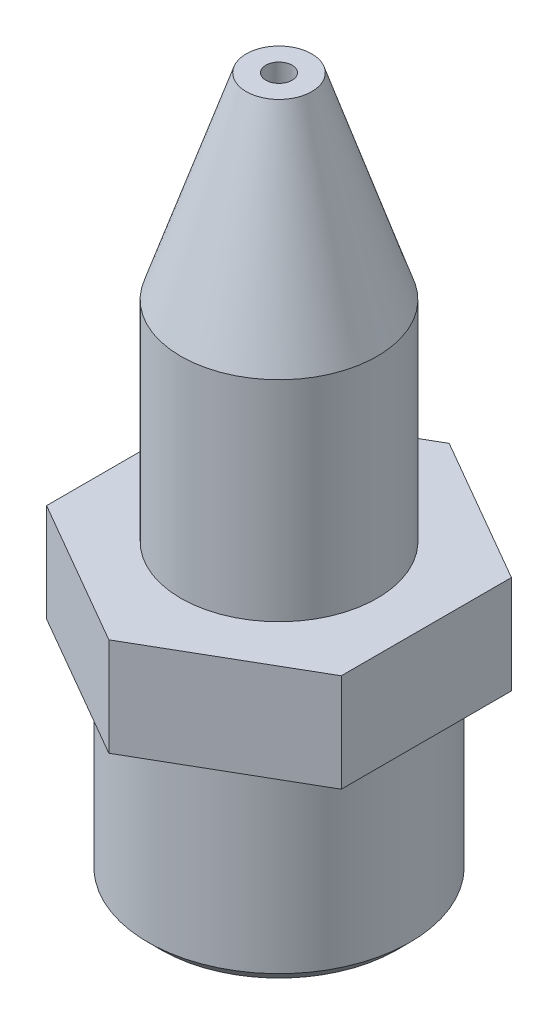
SolidWorks part; units mm, degrees
ref_plane "Front Plane" through (0, 0, 0) normal (0, 0, 1) x (1, 0, 0)
ref_plane "Top Plane" through (0, 0, 0) normal (0, 1, 0) x (1, 0, 0)
ref_plane "Right Plane" through (0, 0, 0) normal (1, 0, 0) x (0, 0, -1)
sketch "Sketch1" plane through (0, 0, 0) normal (0, 1, 0) x (1, 0, 0)
  circle A0 centre (0, 0) radius 1.5
  dimension "D1" = 3
extrude "Boss-Extrude1" add sketch "Sketch1" along normal blind 6.2
sketch "Sketch3" plane through (0, 6.2, 0) normal (0, 1, 0) x (1, 0, 0)
  circle A0 centre (0, 0) radius 0.2
  dimension "D1" = 0.4
extrude "Cut-Extrude2" cut sketch "Sketch3" against normal through all
chamfer "Chamfer1" distance 3 distance2 1 1 edges at (0, 6.2, 1.5)
sketch "Sketch5" plane through (0, 0, 0) normal (0, -1, 0) x (1, 0, 0)
  circle A0 centre (0, 0) radius 0.5
  dimension "D1" = 1
extrude "Cut-Extrude3" cut sketch "Sketch5" against normal blind 1.5
sketch "Sketch7" plane through (0, 0, 0) normal (0, -1, 0) x (1, 0, 0)
  line L1 (0, 2.5981) -> (-2.25, 1.299)
  line L2 (-2.25, 1.299) -> (-2.25, -1.299)
  line L3 (-2.25, -1.299) -> (0, -2.5981)
  line L4 (0, -2.5981) -> (2.25, -1.299)
  line L5 (2.25, -1.299) -> (2.25, 1.299)
  line L6 (2.25, 1.299) -> (0, 2.5981)
  circle A0 centre (0, 0) radius 2.25 construction
  circle A2 centre (0, 0) radius 0.5 construction
  circle A3 centre (0, 0) radius 0.5
  dimension "D1" = 4.5
extrude "Boss-Extrude2" add sketch "Sketch7" along normal blind 1.5
sketch "Sketch8" plane through (0, -1.5, 0) normal (0, -1, 0) x (1, 0, 0)
  circle A2 centre (0, 0) radius 2
  circle A3 centre (0, 0) radius 0.5 construction
  circle A4 centre (0, 0) radius 0.5
  dimension "D1" = 4
extrude "Boss-Extrude3" add sketch "Sketch8" along normal blind 3
cosmetic thread "Cosmetic Thread1" parameters "D2"=3.3
cosmetic thread "Cosmetic Thread2" parameters "D2"=3.3
sketch "Sketch9" plane through (0, 0, 0) normal (0, 0, 1) x (1, 0, 0)
  line L0 (0, -1009.6433) -> (0, -4.8216) construction
  line L2 (0.2, 6.2) -> (1.1, -4.5)
  line L3 (0.2, 6.2) -> (-0.2, 6.2) construction
  line L4 (0.5, 6.2) -> (-0.5, 6.2) construction
  line L5 (-2, -4.5) -> (2, -4.5) construction
  line L6 (0.2, 6.2) -> (0, 6.2)
  line L7 (0, 6.2) -> (0, -4.5)
  line L8 (1.1, -4.5) -> (0, -4.5)
  line L9 (0, -4.5) -> (0, 50000) construction
  dimension "D1" = 2.2
  dimension "D2" = 0.4
revolve "Cut-Revolve2" cut sketch "Sketch9" angle 360 about L0
chamfer "Chamfer4" distance 0.2 angle 45 1 edges at (0, -4.5, -2)
